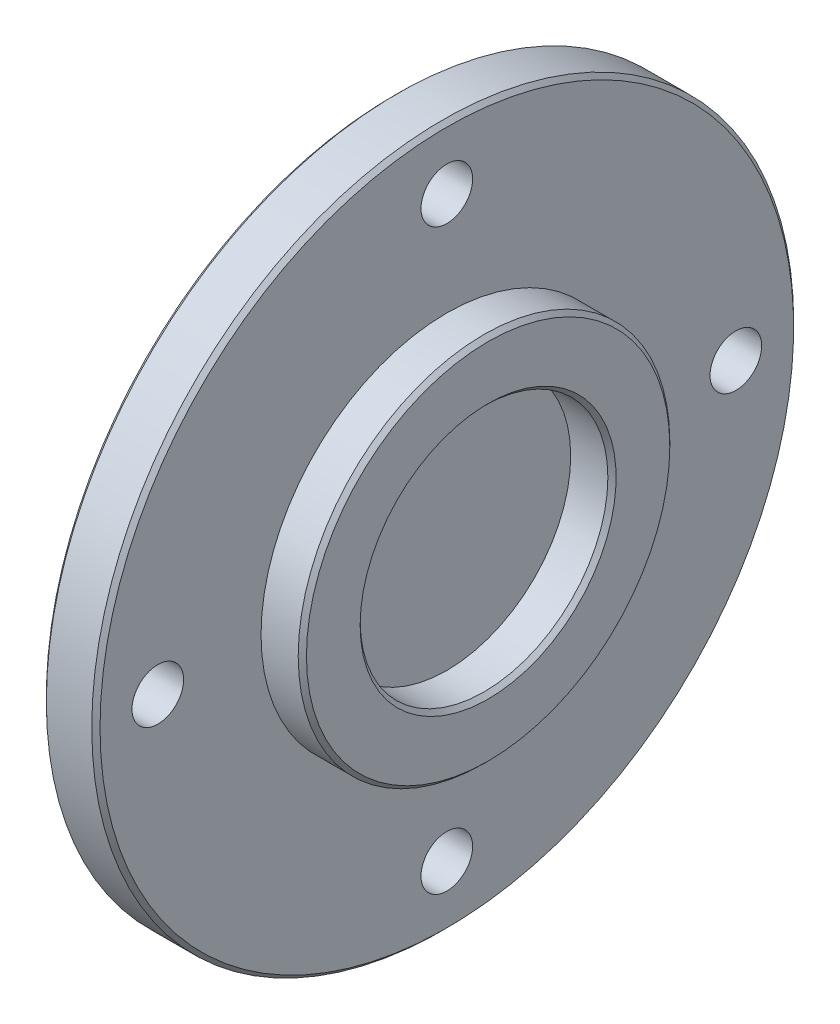
SolidWorks part; units mm, degrees
material "普通碳钢"
ref_plane "前视基准面" through (0, 0, 0) normal (0, 0, 1) x (1, 0, 0)
ref_plane "上视基准面" through (0, 0, 0) normal (0, 1, 0) x (1, 0, 0)
ref_plane "右视基准面" through (0, 0, 0) normal (1, 0, 0) x (0, 0, -1)
sketch "草图1" plane through (0, 0, 0) normal (0, 0, 1) x (1, 0, 0)
  line L0 (0, 0) -> (0, 290.7532) construction
  line L1 (0, 0) -> (356.4696, 0) construction
  line L2 (0, 0) -> (0, 85)
  line L3 (0, 85) -> (13, 85)
  line L4 (13, 85) -> (13, 45)
  line L5 (13, 45) -> (23, 45)
  line L6 (23, 45) -> (23, 30)
  line L7 (23, 30) -> (13, 30)
  line L8 (13, 30) -> (13, 0)
  line L9 (13, 0) -> (0, 0)
  dimension "D1" = 170
  dimension "D2" = 90
  dimension "D3" = 15
  dimension "D4" = 13
  dimension "D5" = 10
revolve "旋转1" add sketch "草图1" angle 360 about L1
sketch "草图2" plane through (0, 0, 0) normal (-1, 0, 0) x (0, 0, 1)
  line L0 (0, 0) -> (0, 70) construction
  circle A0 centre (0, 70) radius 6.25
  dimension "D2" = 12.5
  dimension "D1" = 70
extrude "切除-拉伸1" cut sketch "草图2" against normal through all
pattern_circular "阵列(圆周)1" count 4 over 360 about axis through (0, 0, 0) along (1, 0, 0) of "切除-拉伸1"
chamfer "倒角1" distance 1 angle 45 4 edges at (23, 0, 30) (23, 0, 45) (0, 0, 85) (13, 0, 85)
